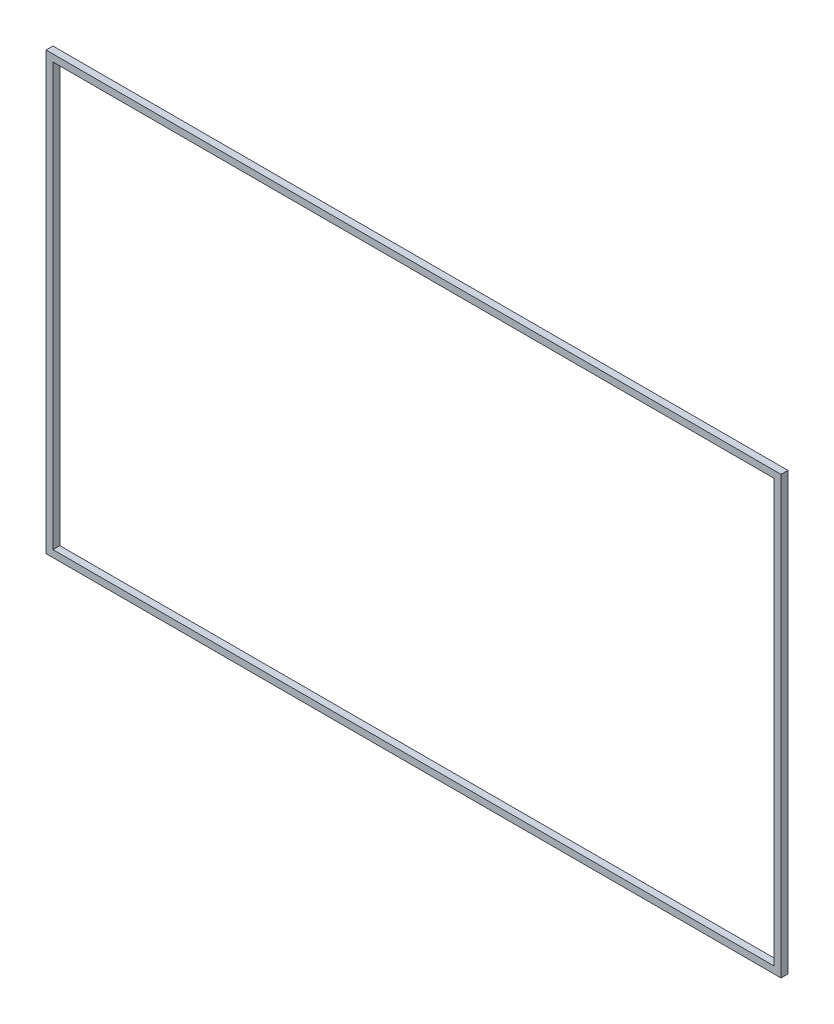
from build123d import *

# Parameters (mm, degrees)
SKETCH_1_W      = 1042
SKETCH_1_H      = 610.2
EXTRUDE_1_DEPTH = 10


with BuildPart() as part:
    # 草图1 → 凸台-拉伸1 (new body)
    with BuildSketch(Plane.XY):
        Polygon((-531, 5), (531, 5), (531, -5), (531, -615.2), (531, -625.2), (-531, -625.2), align=None)
        with Locations((0, -310.1)):
            Rectangle(SKETCH_1_W, SKETCH_1_H, mode=Mode.SUBTRACT)
    extrude(amount=EXTRUDE_1_DEPTH)


solid = part.part
